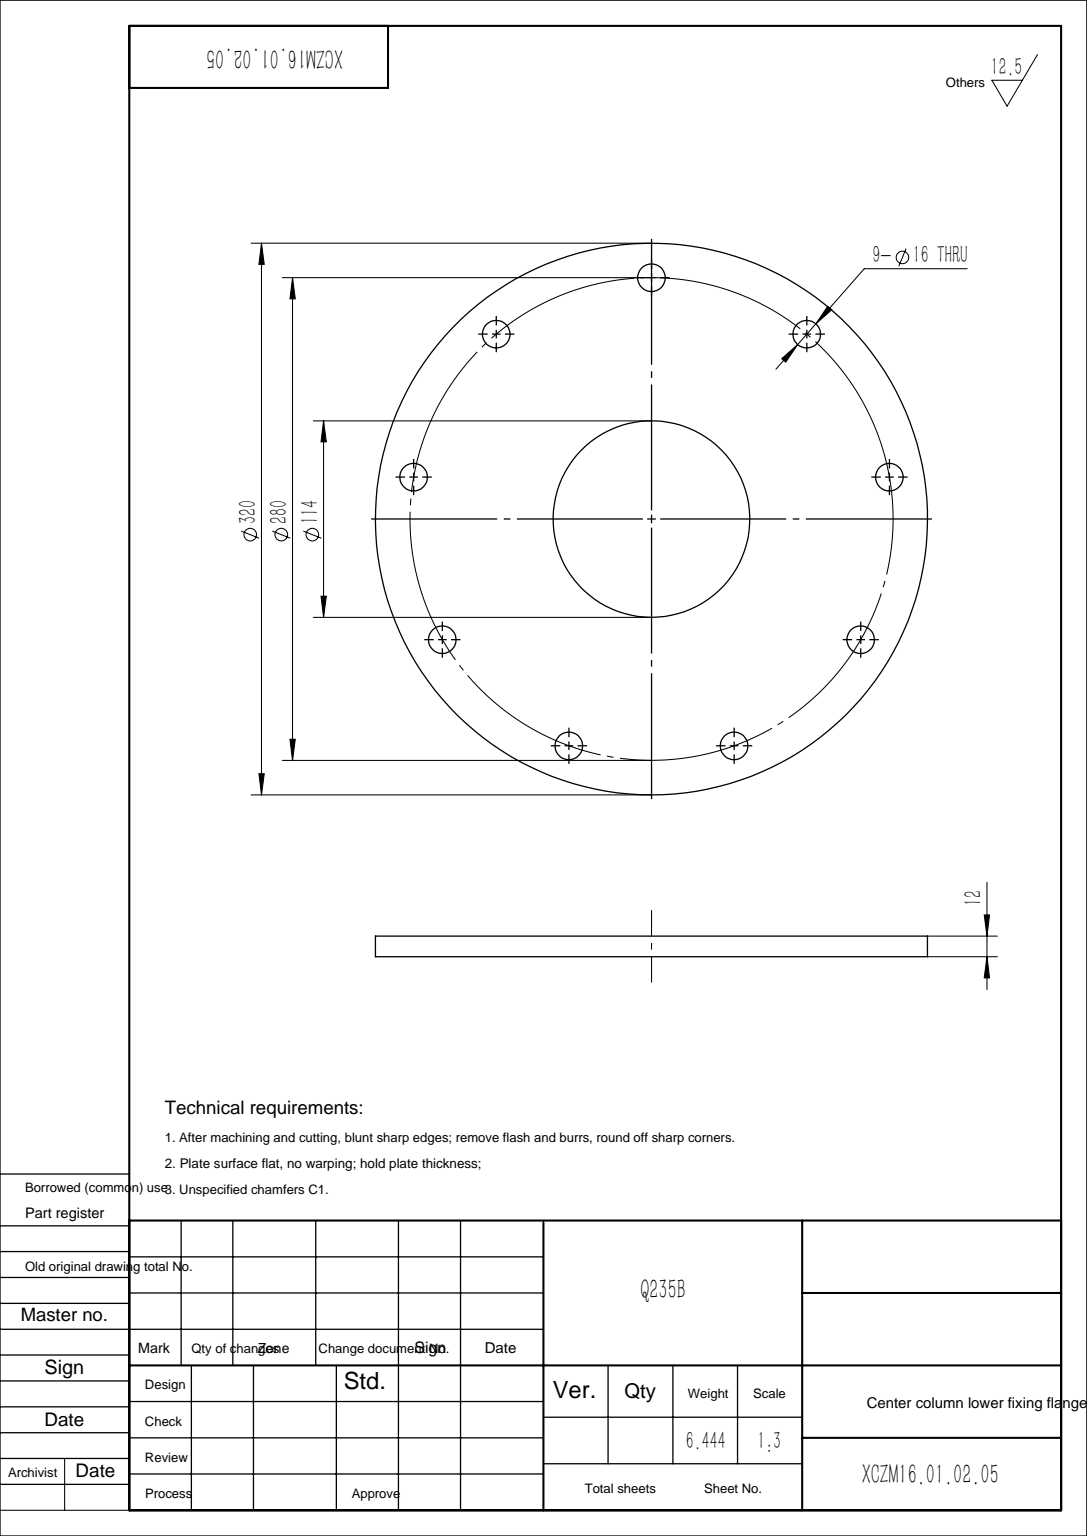
from build123d import *

# Parameters (mm, degrees)
SKETCH1_R           = 160
SKETCH1_R_2         = 57
SKETCH1_R_3         = 8
BOSS_EXTRUDE1_DEPTH = 12


with BuildPart() as part:
    # Sketch1 → Boss-Extrude1 (new body)
    with BuildSketch(Plane(origin=(0, 0, 0), x_dir=(1, 0, 0), z_dir=(0, 1, 0))):
        with Locations(Location((0, 0, 0), (0, 0, 270))):
            Circle(SKETCH1_R)
        with Locations(Location((0, 0, 0), (0, 0, 270))):
            Circle(SKETCH1_R_2, mode=Mode.SUBTRACT)
        with Locations(Location((0, 140, 0), (0, 0, 270))):
            Circle(SKETCH1_R_3, mode=Mode.SUBTRACT)
        with Locations(Location((89.990265356, 107.246222037, 0), (0, 0, 270))):
            Circle(SKETCH1_R_3, mode=Mode.SUBTRACT)
        with Locations(Location((137.873085422, 24.310744873, 0), (0, 0, 270))):
            Circle(SKETCH1_R_3, mode=Mode.SUBTRACT)
        with Locations(Location((121.24355653, -70, 0), (0, 0, 270))):
            Circle(SKETCH1_R_3, mode=Mode.SUBTRACT)
        with Locations(Location((47.882820066, -131.55696691, 0), (0, 0, 270))):
            Circle(SKETCH1_R_3, mode=Mode.SUBTRACT)
        with Locations(Location((-47.882820066, -131.55696691, 0), (0, 0, 270))):
            Circle(SKETCH1_R_3, mode=Mode.SUBTRACT)
        with Locations(Location((-121.24355653, -70, 0), (0, 0, 270))):
            Circle(SKETCH1_R_3, mode=Mode.SUBTRACT)
        with Locations(Location((-137.873085422, 24.310744873, 0), (0, 0, 270))):
            Circle(SKETCH1_R_3, mode=Mode.SUBTRACT)
        with Locations(Location((-89.990265356, 107.246222037, 0), (0, 0, 270))):
            Circle(SKETCH1_R_3, mode=Mode.SUBTRACT)
    extrude(amount=BOSS_EXTRUDE1_DEPTH)


solid = part.part
